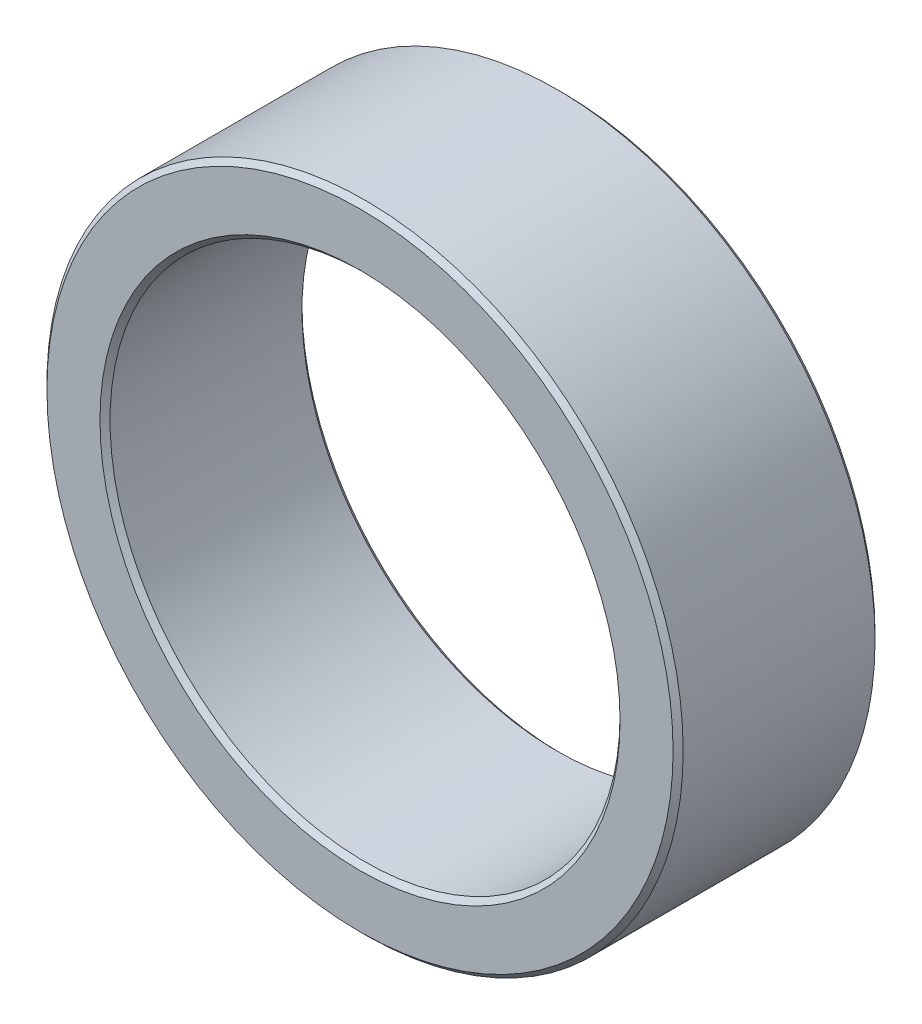
from build123d import *

# Parameters (mm, degrees)
SKETCH_1_R      = 31.5
SKETCH_1_R_2    = 25.25
EXTRUDE_1_DEPTH = 20
CHAMFER_1_SIZE  = 0.5


with BuildPart() as part:
    # 草图1 → 凸台-拉伸1 (new body)
    with BuildSketch(Plane.XY):
        Circle(SKETCH_1_R)
        Circle(SKETCH_1_R_2, mode=Mode.SUBTRACT)
    extrude(amount=EXTRUDE_1_DEPTH)

    # 倒角1
    chamfer_1_edges = [part.edges().sort_by_distance(p)[0] for p in [
        (-31.5, 0, 0),
        (-31.5, 0, 20),
        (-25.25, 0, 0),
        (-25.25, 0, 20),
    ]]
    chamfer(chamfer_1_edges, length=CHAMFER_1_SIZE)


solid = part.part
